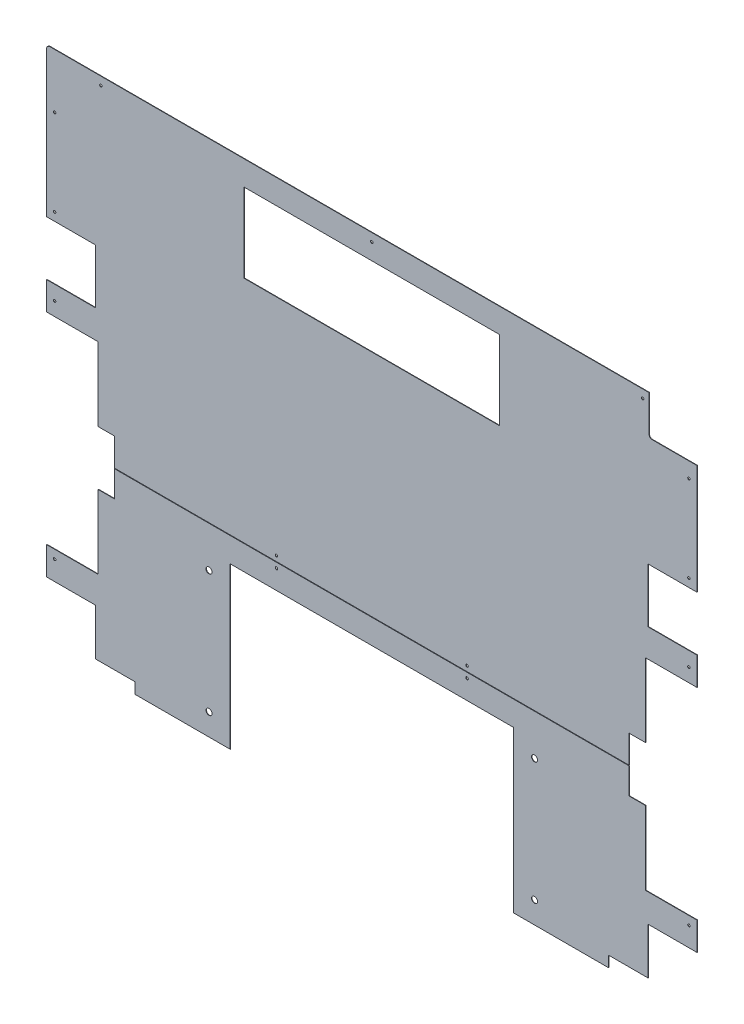
from build123d import *

# Parameters (mm, degrees)
SKETCH_1_W             = 1195
SKETCH_1_H             = 1360
EXTRUDE_1_DEPTH        = 0.8
SKETCH_2_W             = 190
SKETCH_2_H             = 370
CUT_EXTRUDE_2618_DEPTH = 959.909218852
FILLET_6_R             = 6.5
FILLET_7_R             = 6.5
SKETCH_3_W             = 470
SKETCH_3_H             = 145
CUT_EXTRUDE_3491_DEPTH = 10
SKETCH_8_R             = 5.5
SKETCH_8_W             = 520
SKETCH_8_H             = 295
CUT_EXTRUDE_4077_DEPTH = 959.909218852
SKETCH_4_W             = 60
SKETCH_4_H             = 100
CUT_EXTRUDE_4742_DEPTH = 10
SKETCH_5_R             = 2.25
CUT_EXTRUDE_5780_DEPTH = 10
SKETCH_7_W             = 90
SKETCH_7_H             = 100
CUT_EXTRUDE_6423_DEPTH = 10
SKETCH_17_R            = 2.25
CUT_EXTRUDE_4_DEPTH    = 959.909218852
CUT_EXTRUDE_7850_REACH = 960.909
SKETCH_18_W            = 1195
SKETCH_18_H            = 408
SKETCH_19_W            = 162.5
SKETCH_19_H            = 20
CUT_EXTRUDE_8511_DEPTH = 854.877561481
CUT_EXTRUDE_1_DEPTH    = 10
SKETCH_21_R            = 2.25
CUT_EXTRUDE_2_DEPTH    = 10
SKETCH_22_W            = 1215
SKETCH_22_H            = 1
CUT_EXTRUDE_4_2_DEPTH  = 10
SKETCH_23_R            = 2.25
CUT_EXTRUDE_5_DEPTH    = 20


with BuildPart() as part:
    # 草图1 → 凸台-拉伸1 (new body)
    with BuildSketch(Plane.XY):
        with Locations((0, -70)):
            Rectangle(SKETCH_1_W, SKETCH_1_H)
    extrude(amount=EXTRUDE_1_DEPTH)

    # 草图2 → Cut-Extrude 2618 (cut, through all)
    with BuildSketch(Plane.XY.offset(0.8)):
        with Locations((-597.5, 0)):
            Rectangle(SKETCH_2_W, SKETCH_2_H)
        with Locations((597.5, 0)):
            Rectangle(SKETCH_2_W, SKETCH_2_H)
    extrude(amount=-CUT_EXTRUDE_2618_DEPTH, mode=Mode.SUBTRACT)

    # 圆角6
    fillet_6_edges = [part.edges().sort_by_distance(p)[0] for p in [
        (-597.5, 610, 0.4),
    ]]
    fillet(fillet_6_edges, radius=FILLET_6_R)

    # 圆角7
    fillet_7_edges = [part.edges().sort_by_distance(p)[0] for p in [
        (597.5, 610, 0.4),
    ]]
    fillet(fillet_7_edges, radius=FILLET_7_R)

    # 草图3 → Cut-Extrude 3491 (cut)
    with BuildSketch(Plane.XY.offset(0.8)):
        with Locations((0, 492.5)):
            Rectangle(SKETCH_3_W, SKETCH_3_H)
    extrude(amount=-CUT_EXTRUDE_3491_DEPTH, mode=Mode.SUBTRACT)

    # 草图8 → Cut-Extrude 4077 (cut, through all)
    with BuildSketch(Plane(origin=(0, 0, 0), x_dir=(-1, 0, 0), z_dir=(0, 0, -1))):
        with Locations((-299, -77)):
            Circle(SKETCH_8_R)
        with Locations((-299, -302)):
            Circle(SKETCH_8_R)
        with Locations(Location((299, -302, 0), (0, 0, 180))):
            Circle(SKETCH_8_R)
        with Locations(Location((299, -77, 0), (0, 0, 180))):
            Circle(SKETCH_8_R)
        with Locations((0, -194.5)):
            Rectangle(SKETCH_8_W, SKETCH_8_H)
    extrude(amount=-CUT_EXTRUDE_4077_DEPTH, mode=Mode.SUBTRACT)

    # 草图4 → Cut-Extrude 4742 (cut)
    with BuildSketch(Plane.XY.offset(0.8)):
        with Locations((-502.5, 0)):
            Rectangle(SKETCH_4_W, SKETCH_4_H)
        with Locations((502.5, 0)):
            Rectangle(SKETCH_4_W, SKETCH_4_H)
    extrude(amount=-CUT_EXTRUDE_4742_DEPTH, mode=Mode.SUBTRACT)

    # 草图5 → Cut-Extrude 5780 (cut)
    with BuildSketch(Plane.XY.offset(0.8)):
        with Locations((-497.5, 595)):
            Circle(SKETCH_5_R)
        with Locations((-582.5, 510)):
            Circle(SKETCH_5_R)
        with Locations((582.5, 510)):
            Circle(SKETCH_5_R)
        with Locations((497.5, 595)):
            Circle(SKETCH_5_R)
        with Locations((0, 595)):
            Circle(SKETCH_5_R)
        with Locations((-582.5, 210)):
            Circle(SKETCH_5_R)
        with Locations((582.5, 210)):
            Circle(SKETCH_5_R)
    extrude(amount=-CUT_EXTRUDE_5780_DEPTH, mode=Mode.SUBTRACT)

    # 草图7 → Cut-Extrude 6423 (cut)
    with BuildSketch(Plane(origin=(0, 0, 0), x_dir=(-1, 0, 0), z_dir=(0, 0, -1))):
        with Locations((552.5, -286.5)):
            Rectangle(SKETCH_7_W, SKETCH_7_H)
        with Locations((-552.5, 286.5)):
            Rectangle(SKETCH_7_W, SKETCH_7_H)
        with Locations((552.5, 286.5)):
            Rectangle(SKETCH_7_W, SKETCH_7_H)
        with Locations((-552.5, -286.5)):
            Rectangle(SKETCH_7_W, SKETCH_7_H)
    extrude(amount=-CUT_EXTRUDE_6423_DEPTH, mode=Mode.SUBTRACT)

    # 草图17 → Cut-Extrude 4 (cut, through all)
    with BuildSketch(Plane(origin=(0, 0, 0), x_dir=(-1, 0, 0), z_dir=(0, 0, -1))):
        with Locations((-582.5, -200.75)):
            Circle(SKETCH_17_R)
        with Locations(Location((582.5, -200.75, 0), (0, 0, 180))):
            Circle(SKETCH_17_R)
    extrude(amount=-CUT_EXTRUDE_4_DEPTH, mode=Mode.SUBTRACT)

    # 草图18 → Cut-Extrude 7850 (cut, up to next)
    with BuildSketch(Plane(origin=(0, 0, 0), x_dir=(-1, 0, 0), z_dir=(0, 0, -1)), mode=Mode.PRIVATE) as cut_extrude_7850_sk1:
        with Locations((0, -546)):
            Rectangle(SKETCH_18_W, SKETCH_18_H)
    cut_extrude_7850_tool1 = extrude(cut_extrude_7850_sk1.sketch, amount=-CUT_EXTRUDE_7850_REACH, mode=Mode.PRIVATE) & part.part
    add(cut_extrude_7850_tool1.solids().sort_by_distance((0, -546, 0))[0], mode=Mode.SUBTRACT)

    # 草图19 → Cut-Extrude 8511 (cut, through all)
    with BuildSketch(Plane(origin=(0, 0, 0), x_dir=(-1, 0, 0), z_dir=(0, 0, -1))):
        with Locations((-516.25, -332)):
            Rectangle(SKETCH_19_W, SKETCH_19_H)
        with Locations((516.25, -332)):
            Rectangle(SKETCH_19_W, SKETCH_19_H)
    extrude(amount=-CUT_EXTRUDE_8511_DEPTH, mode=Mode.SUBTRACT)

    # 草图20 → Cut-Extrude 1 (cut)
    with BuildSketch(Plane(origin=(0, 0, 0), x_dir=(-1, 0, 0), z_dir=(0, 0, -1))):
        with BuildLine():
            Line((-597.5, 610), (-509.5, 610))
            Line((-509.5, 610), (-509.5, 543))
            ThreePointArc((-509.5, 543), (-510.964466094, 539.464466094), (-514.5, 538))
            Line((-514.5, 538), (-597.5, 538))
            Line((-597.5, 538), (-597.5, 610))
        make_face()
    extrude(amount=-CUT_EXTRUDE_1_DEPTH, mode=Mode.SUBTRACT)

    # 草图21 → Cut-Extrude 2 (cut)
    with BuildSketch(Plane(origin=(0, 0, 0), x_dir=(-1, 0, 0), z_dir=(0, 0, -1))):
        with Locations((-582.5, 351.5)):
            Circle(SKETCH_21_R)
        with Locations(Location((582.5, 351.5, 0), (0, 0, 180))):
            Circle(SKETCH_21_R)
    extrude(amount=-CUT_EXTRUDE_2_DEPTH, mode=Mode.SUBTRACT)

    # 草图22 → Cut-Extrude 4 2 (cut)
    with BuildSketch(Plane(origin=(0, 0, 0), x_dir=(-1, 0, 0), z_dir=(0, 0, -1))):
        with Locations((0, -1.5)):
            Rectangle(SKETCH_22_W, SKETCH_22_H)
    extrude(amount=-CUT_EXTRUDE_4_2_DEPTH, mode=Mode.SUBTRACT)


with BuildPart() as cut_extrude_4_2_piece_1:
    # of the separate pieces the step leaves, piece 1, a body of its own (cut_extrude_4_2_pieces)
    add(part.part.solids().sort_by_distance((-591, 610, 0))[0])


with BuildPart() as cut_extrude_4_2_piece_2:
    # of the separate pieces the step leaves, piece 2, a body of its own (cut_extrude_4_2_pieces)
    add(part.part.solids().sort_by_distance((-472.5, -2, 0))[0])


with BuildPart() as cut_extrude_5_tool:
    # 草图23 → 切除-拉伸5 (new body)
    with BuildSketch(Plane(origin=(0, 0, 0), x_dir=(-1, 0, 0), z_dir=(0, 0, -1))):
        with Locations((-175, -11.5)):
            Circle(SKETCH_23_R)
        with Locations(Location((175, -11.5, 0), (0, 0, 180))):
            Circle(SKETCH_23_R)
        with Locations((-175, 8.5)):
            Circle(SKETCH_23_R)
        with Locations(Location((175, 8.5, 0), (0, 0, 180))):
            Circle(SKETCH_23_R)
    extrude(amount=-CUT_EXTRUDE_5_DEPTH)


with BuildPart() as cut_extrude_4_2_piece_1_1:
    add(cut_extrude_4_2_piece_1.part)

    # 切除-拉伸5: cut by cut_extrude_5_tool
    add(cut_extrude_5_tool.part, mode=Mode.SUBTRACT)


with BuildPart() as cut_extrude_4_2_piece_2_1:
    add(cut_extrude_4_2_piece_2.part)

    # 切除-拉伸5: cut by cut_extrude_5_tool
    add(cut_extrude_5_tool.part, mode=Mode.SUBTRACT)


solid = Compound([cut_extrude_4_2_piece_1_1.part, cut_extrude_4_2_piece_2_1.part])
